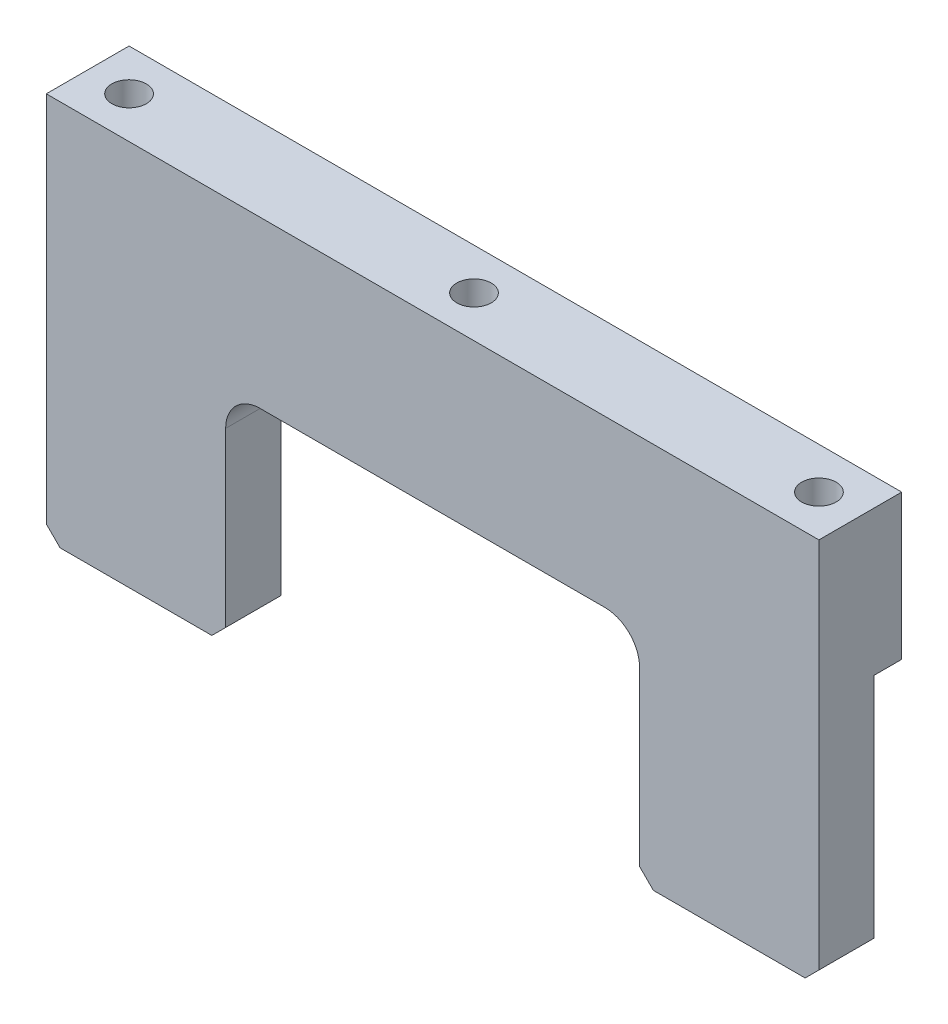
from build123d import *

# Parameters (mm, degrees)
SKETCH1_W             = 112
SKETCH1_H             = 56
BOSS_EXTRUDE1_DEPTH   = 12
SKETCH2_W             = 112
SKETCH2_H             = 35
CUT_EXTRUDE1_DEPTH    = 4
M6_TAPPED_HOLE1_D     = 5
M6_TAPPED_HOLE1_DEPTH = 15
M6_TAPPED_HOLE1_TIP   = 1.502151548
SKETCH6_W             = 60
SKETCH6_H             = 32
CUT_EXTRUDE2_DEPTH    = 126.475097131
FILLET1_R             = 5
CHAMFER1_SIZE         = 2


with BuildPart() as part:
    # Sketch1 → Boss-Extrude1 (new body)
    with BuildSketch(Plane.XY):
        with Locations((56, 28)):
            Rectangle(SKETCH1_W, SKETCH1_H)
    extrude(amount=BOSS_EXTRUDE1_DEPTH)

    # Sketch2 → Cut-Extrude1 (cut)
    with BuildSketch(Plane(origin=(0, 0, 0), x_dir=(-1, 0, 0), z_dir=(0, 0, -1))):
        with Locations((-56, 17.5)):
            Rectangle(SKETCH2_W, SKETCH2_H)
    extrude(amount=-CUT_EXTRUDE1_DEPTH, mode=Mode.SUBTRACT)

    # M6 Tapped Hole1
    with Locations(Plane(origin=(0, 56, 0), x_dir=(1, 0, 0), z_dir=(0, 1, 0))):
        with Locations((106, -6), (6, -6), (56, -6)):
            Hole(M6_TAPPED_HOLE1_D / 2, depth=M6_TAPPED_HOLE1_DEPTH)
            with Locations((0, 0, -(M6_TAPPED_HOLE1_DEPTH + M6_TAPPED_HOLE1_TIP / 2))):  # 118° drill point
                Cone(0, M6_TAPPED_HOLE1_D / 2, M6_TAPPED_HOLE1_TIP, mode=Mode.SUBTRACT)

    # Sketch6 → Cut-Extrude2 (cut, through all)
    with BuildSketch(Plane(origin=(0, 0, 4), x_dir=(-1, 0, 0), z_dir=(0, 0, -1))):
        with Locations((-56, 16)):
            Rectangle(SKETCH6_W, SKETCH6_H)
    extrude(amount=-CUT_EXTRUDE2_DEPTH, mode=Mode.SUBTRACT)

    # Fillet1
    fillet1_edges = [part.edges().sort_by_distance(p)[0] for p in [
        (86, 32, 8),
        (26, 32, 8),
    ]]
    fillet(fillet1_edges, radius=FILLET1_R)

    # Chamfer1
    chamfer1_edges = [part.edges().sort_by_distance(p)[0] for p in [
        (86, 0, 8),
        (26, 0, 8),
        (112, 0, 8),
        (0, 0, 8),
    ]]
    chamfer(chamfer1_edges, length=CHAMFER1_SIZE)


solid = part.part
